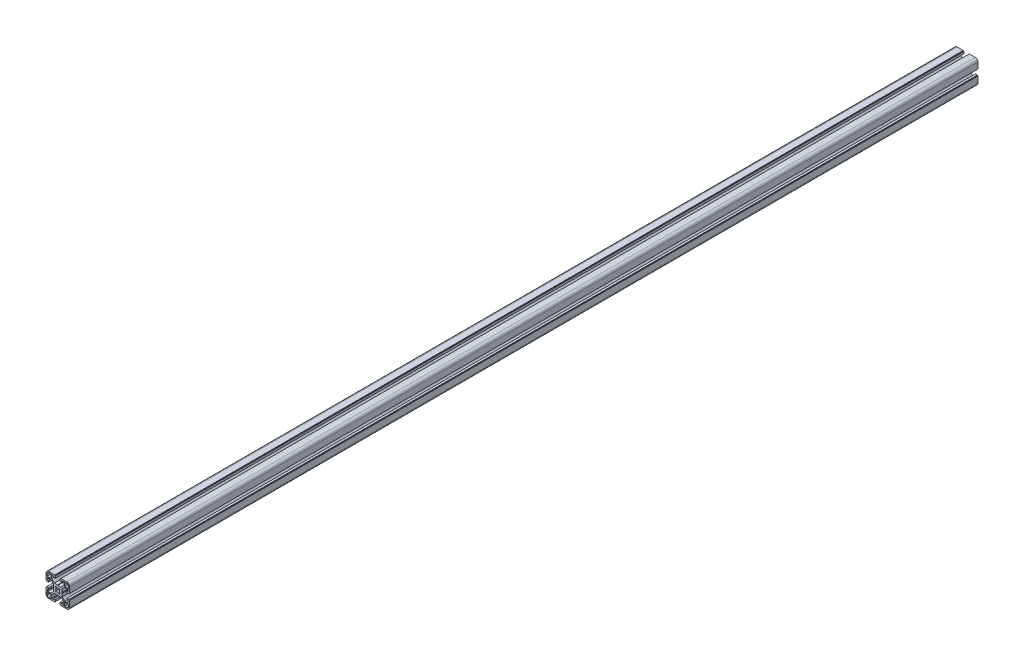
from build123d import *

# Parameters (mm, degrees)
EXTRUDE_1_DEPTH = 1548


with BuildPart() as part:
    # 草图1 → 凸台-拉伸1 (new body)
    with BuildSketch(Plane.XY):
        with BuildLine():
            Line((-18.9995, -4.100341675), (-18.9995, -5.100341675))
            Line((-18.9995, -5.100341675), (-19.9995, -5.100341675))
            Line((-19.9995, -5.100341675), (-19.9995, -15.500341675))
            ThreePointArc((-19.9995, -15.500341675), (-18.681480515, -18.682322191), (-15.4995, -20.000341675))
            Line((-15.4995, -20.000341675), (-5.0995, -20.000341675))
            Line((-5.0995, -20.000341675), (-5.0995, -19.000341675))
            Line((-5.0995, -19.000341675), (-4.0995, -19.000341675))
            Line((-4.0995, -19.000341675), (-4.0995, -15.500341675))
            Line((-4.0995, -15.500341675), (-6.5995, -15.500341675))
            Line((-6.5995, -15.500341675), (-6.5995, -16.500341675))
            ThreePointArc((-6.5995, -16.500341675), (-6.892393219, -17.207448457), (-7.5995, -17.500341675))
            Line((-7.5995, -17.500341675), (-9.7995, -17.500341675))
            ThreePointArc((-9.7995, -17.500341675), (-10.153053391, -17.353895066), (-10.2995, -17.000341675))
            Line((-10.2995, -17.000341675), (-10.2995, -11.997341675))
            Line((-10.2995, -11.997341675), (-5.9025, -7.600341675))
            Line((-5.9025, -7.600341675), (-0.5195, -7.600341675))
            Line((-0.5195, -7.600341675), (0.0005, -7.300341675))
            Line((0.0005, -7.300341675), (0.5195, -7.600341675))
            Line((0.5195, -7.600341675), (5.9035, -7.600341675))
            Line((5.9035, -7.600341675), (10.3005, -11.997341675))
            Line((10.3005, -11.997341675), (10.3005, -17.000341675))
            ThreePointArc((10.3005, -17.000341675), (10.154053391, -17.353895066), (9.8005, -17.500341675))
            Line((9.8005, -17.500341675), (7.6005, -17.500341675))
            ThreePointArc((7.6005, -17.500341675), (6.893393219, -17.207448457), (6.6005, -16.500341675))
            Line((6.6005, -16.500341675), (6.6005, -15.500341675))
            Line((6.6005, -15.500341675), (4.1005, -15.500341675))
            Line((4.1005, -15.500341675), (4.1005, -19.000341675))
            Line((4.1005, -19.000341675), (5.1005, -19.000341675))
            Line((5.1005, -19.000341675), (5.1005, -20.000341675))
            Line((5.1005, -20.000341675), (15.5005, -20.000341675))
            ThreePointArc((15.5005, -20.000341675), (18.682480515, -18.682322191), (20.0005, -15.500341675))
            Line((20.0005, -15.500341675), (20.0005, -5.100341675))
            Line((20.0005, -5.100341675), (19.0005, -5.100341675))
            Line((19.0005, -5.100341675), (19.0005, -4.100341675))
            Line((19.0005, -4.100341675), (15.5005, -4.100341675))
            Line((15.5005, -4.100341675), (15.5005, -6.600341675))
            Line((15.5005, -6.600341675), (16.5005, -6.600341675))
            ThreePointArc((16.5005, -6.600341675), (17.207606781, -6.893234894), (17.5005, -7.600341675))
            Line((17.5005, -7.600341675), (17.5005, -9.800341675))
            ThreePointArc((17.5005, -9.800341675), (17.354053391, -10.153895066), (17.0005, -10.300341675))
            Line((17.0005, -10.300341675), (11.9975, -10.300341675))
            Line((11.9975, -10.300341675), (7.6005, -5.903341675))
            Line((7.6005, -5.903341675), (7.6005, -0.520341675))
            Line((7.6005, -0.520341675), (7.3005, -0.000341675))
            Line((7.3005, -0.000341675), (7.6005, 0.519658325))
            Line((7.6005, 0.519658325), (7.6005, 5.902658325))
            Line((7.6005, 5.902658325), (11.9975, 10.299658325))
            Line((11.9975, 10.299658325), (17.0005, 10.299658325))
            ThreePointArc((17.0005, 10.299658325), (17.354053391, 10.153211715), (17.5005, 9.799658325))
            Line((17.5005, 9.799658325), (17.5005, 7.599658325))
            ThreePointArc((17.5005, 7.599658325), (17.207606781, 6.892551543), (16.5005, 6.599658325))
            Line((16.5005, 6.599658325), (15.5005, 6.599658325))
            Line((15.5005, 6.599658325), (15.5005, 4.099658325))
            Line((15.5005, 4.099658325), (19.0005, 4.099658325))
            Line((19.0005, 4.099658325), (19.0005, 5.099658325))
            Line((19.0005, 5.099658325), (20.0005, 5.099658325))
            Line((20.0005, 5.099658325), (20.0005, 15.499658325))
            ThreePointArc((20.0005, 15.499658325), (18.682480515, 18.68163884), (15.5005, 19.999658325))
            Line((15.5005, 19.999658325), (5.1005, 19.999658325))
            Line((5.1005, 19.999658325), (5.1005, 18.999658325))
            Line((5.1005, 18.999658325), (4.1005, 18.999658325))
            Line((4.1005, 18.999658325), (4.1005, 15.499658325))
            Line((4.1005, 15.499658325), (6.6005, 15.499658325))
            ThreePointArc((6.6005, 15.499658325), (6.393348977, 15.999658325), (6.6005, 16.499658325))
            ThreePointArc((6.6005, 16.499658325), (6.893393219, 17.206765106), (7.6005, 17.499658325))
            Line((7.6005, 17.499658325), (9.8005, 17.499658325))
            ThreePointArc((9.8005, 17.499658325), (10.154053391, 17.353211715), (10.3005, 16.999658325))
            Line((10.3005, 16.999658325), (10.3005, 11.996658325))
            Line((10.3005, 11.996658325), (5.9035, 7.599658325))
            Line((5.9035, 7.599658325), (0.5195, 7.599658325))
            Line((0.5195, 7.599658325), (0.0005, 7.299658325))
            Line((0.0005, 7.299658325), (-0.5195, 7.599658325))
            Line((-0.5195, 7.599658325), (-5.9025, 7.599658325))
            Line((-5.9025, 7.599658325), (-10.2995, 11.996658325))
            Line((-10.2995, 11.996658325), (-10.2995, 16.999658325))
            ThreePointArc((-10.2995, 16.999658325), (-10.153053391, 17.353211715), (-9.7995, 17.499658325))
            Line((-9.7995, 17.499658325), (-7.5995, 17.499658325))
            ThreePointArc((-7.5995, 17.499658325), (-6.892393219, 17.206765106), (-6.5995, 16.499658325))
            Line((-6.5995, 16.499658325), (-6.5995, 15.499658325))
            Line((-6.5995, 15.499658325), (-4.0995, 15.499658325))
            Line((-4.0995, 15.499658325), (-4.0995, 18.999658325))
            Line((-4.0995, 18.999658325), (-5.0995, 18.999658325))
            Line((-5.0995, 18.999658325), (-5.0995, 19.999658325))
            Line((-5.0995, 19.999658325), (-15.4995, 19.999658325))
            ThreePointArc((-15.4995, 19.999658325), (-18.681480515, 18.68163884), (-19.9995, 15.499658325))
            Line((-19.9995, 15.499658325), (-19.9995, 5.099658325))
            Line((-19.9995, 5.099658325), (-18.9995, 5.099658325))
            Line((-18.9995, 5.099658325), (-18.9995, 4.099658325))
            Line((-18.9995, 4.099658325), (-15.4995, 4.099658325))
            Line((-15.4995, 4.099658325), (-15.4995, 6.599658325))
            Line((-15.4995, 6.599658325), (-16.4995, 6.599658325))
            ThreePointArc((-16.4995, 6.599658325), (-17.206606781, 6.892551543), (-17.4995, 7.599658325))
            Line((-17.4995, 7.599658325), (-17.4995, 9.799658325))
            ThreePointArc((-17.4995, 9.799658325), (-17.353053391, 10.153211715), (-16.9995, 10.299658325))
            Line((-16.9995, 10.299658325), (-11.9965, 10.299658325))
            Line((-11.9965, 10.299658325), (-7.5995, 5.902658325))
            Line((-7.5995, 5.902658325), (-7.5995, 0.519658325))
            Line((-7.5995, 0.519658325), (-7.2995, -0.000341675))
            Line((-7.2995, -0.000341675), (-7.5995, -0.520341675))
            Line((-7.5995, -0.520341675), (-7.5995, -5.903341675))
            Line((-7.5995, -5.903341675), (-11.9965, -10.300341675))
            Line((-11.9965, -10.300341675), (-16.9995, -10.300341675))
            ThreePointArc((-16.9995, -10.300341675), (-17.353053391, -10.153895066), (-17.4995, -9.800341675))
            Line((-17.4995, -9.800341675), (-17.4995, -7.600341675))
            ThreePointArc((-17.4995, -7.600341675), (-17.206606781, -6.893234894), (-16.4995, -6.600341675))
            Line((-16.4995, -6.600341675), (-15.4995, -6.600341675))
            Line((-15.4995, -6.600341675), (-15.4995, -4.100341675))
            Line((-15.4995, -4.100341675), (-18.9995, -4.100341675))
        make_face()
        with BuildLine():
            Line((15.5005, -18.000341675), (11.8005, -18.000341675))
            Line((11.8005, -18.000341675), (11.8005, -11.800341675))
            Line((11.8005, -11.800341675), (18.0005, -11.800341675))
            Line((18.0005, -11.800341675), (18.0005, -15.500341675))
            ThreePointArc((18.0005, -15.500341675), (17.268266953, -17.268108628), (15.5005, -18.000341675))
        make_face(mode=Mode.SUBTRACT)
        with BuildLine():
            Line((18.0005, 11.799658325), (11.8005, 11.799658325))
            Line((11.8005, 11.799658325), (11.8005, 17.999658325))
            Line((11.8005, 17.999658325), (15.5005, 17.999658325))
            ThreePointArc((15.5005, 17.999658325), (17.268266953, 17.267425278), (18.0005, 15.499658325))
            Line((18.0005, 15.499658325), (18.0005, 11.799658325))
        make_face(mode=Mode.SUBTRACT)
        with BuildLine():
            Line((-1.8145, -2.875341675), (-3.004391671, -4.066450004))
            Line((-3.004391671, -4.066450004), (-4.065608329, -3.005233346))
            Line((-4.065608329, -3.005233346), (-2.8745, -1.815341675))
            ThreePointArc((-2.8745, -1.815341675), (-3.399473913, -0.000341675), (-2.8745, 1.814658325))
            Line((-2.8745, 1.814658325), (-4.064391671, 3.005766654))
            Line((-4.064391671, 3.005766654), (-3.004391671, 4.065766654))
            Line((-3.004391671, 4.065766654), (-1.8145, 2.874658325))
            ThreePointArc((-1.8145, 2.874658325), (0, 3.399316649), (1.8145, 2.874658325))
            Line((1.8145, 2.874658325), (3.0055, 4.065658325))
            Line((3.0055, 4.065658325), (4.066608329, 3.004549996))
            Line((4.066608329, 3.004549996), (2.8755, 1.814658325))
            ThreePointArc((2.8755, 1.814658325), (3.400473913, -0.000341675), (2.8755, -1.815341675))
            Line((2.8755, -1.815341675), (4.066608329, -3.005233346))
            Line((4.066608329, -3.005233346), (3.0055, -4.066341675))
            Line((3.0055, -4.066341675), (1.8145, -2.875341675))
            ThreePointArc((1.8145, -2.875341675), (0, -3.4), (-1.8145, -2.875341675))
        make_face(mode=Mode.SUBTRACT)
        with BuildLine():
            Line((-17.9995, -15.500341675), (-17.9995, -11.800341675))
            Line((-17.9995, -11.800341675), (-11.7995, -11.800341675))
            Line((-11.7995, -11.800341675), (-11.7995, -18.000341675))
            Line((-11.7995, -18.000341675), (-15.4995, -18.000341675))
            ThreePointArc((-15.4995, -18.000341675), (-17.267266953, -17.268108628), (-17.9995, -15.500341675))
        make_face(mode=Mode.SUBTRACT)
        with BuildLine():
            Line((-11.7995, 17.999658325), (-11.7995, 11.799658325))
            Line((-11.7995, 11.799658325), (-17.9995, 11.799658325))
            Line((-17.9995, 11.799658325), (-17.9995, 15.499658325))
            ThreePointArc((-17.9995, 15.499658325), (-17.267266953, 17.267425278), (-15.4995, 17.999658325))
            Line((-15.4995, 17.999658325), (-11.7995, 17.999658325))
        make_face(mode=Mode.SUBTRACT)
    extrude(amount=-EXTRUDE_1_DEPTH)


solid = part.part
